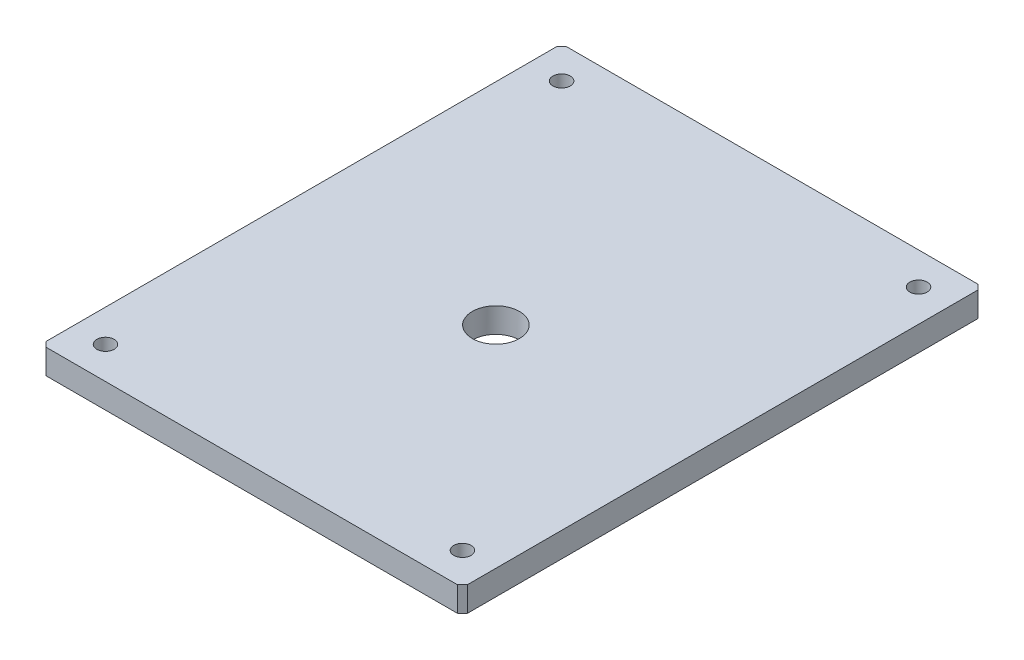
SolidWorks part; units mm, degrees
ref_plane "前视基准面" through (0, 0, 0) normal (0, 0, 1) x (1, 0, 0)
ref_plane "上视基准面" through (0, 0, 0) normal (0, 1, 0) x (1, 0, 0)
ref_plane "右视基准面" through (0, 0, 0) normal (1, 0, 0) x (0, 0, -1)
sketch "草图1" plane through (0, 0, 0) normal (0, 1, 0) x (1, 0, 0)
  line L1 (-85, -105) -> (85, -105)
  line L2 (-85, -105) -> (-85, 105)
  line L3 (-85, 105) -> (85, 105)
  line L4 (85, -105) -> (85, 105)
  line L5 (-85, -105) -> (85, 105) construction
  line L6 (-85, 105) -> (85, -105) construction
  point P0 (0, 0)
  dimension "D1" = 210
  dimension "D2" = 170
extrude "凸台-拉伸1" add sketch "草图1" along normal blind 10
sketch "草图2" plane through (0, 10, 0) normal (0, 1, 0) x (1, 0, 0)
  circle A0 centre (0, -6.5) radius 9.5
  dimension "D1" = 19
extrude "切除-拉伸1" cut sketch "草图2" against normal up to next
sketch "草图3" plane through (0, 0, 0) normal (0, -1, 0) x (1, 0, 0)
  line L0 (85, 105) -> (85, -105) construction
  line L1 (-85, 105) -> (85, 105) construction
  circle A0 centre (72, 92) radius 3.5
  point P2 (61.0905, 77.3444)
  dimension "D1" = 7
  dimension "D2" = 13
  dimension "D3" = 13
extrude "切除-拉伸2" cut sketch "草图3" against normal up to next
mirror "镜向1" about plane through (0, 0, 0) normal (1, 0, 0) of "切除-拉伸2"
mirror "镜向2" about plane through (0, 0, 0) normal (0, 0, 1) of "镜向1", "切除-拉伸2"
chamfer "倒角1" distance 2 angle 45 4 edges at (-85, 5, 105) (-85, 5, -105) (85, 5, -105) (85, 5, 105)
